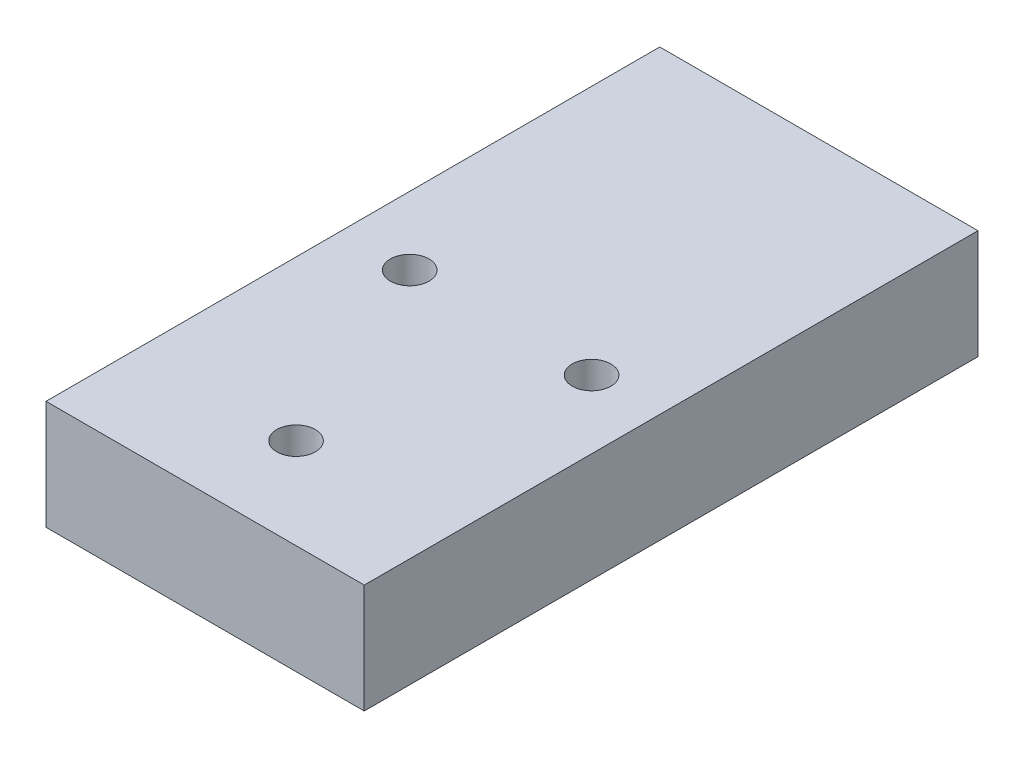
from build123d import *

# Parameters (mm, degrees)
SKETCH_1_W          = 70
SKETCH_1_H          = 135
EXTRUDE_1_DEPTH     = 24
HOLE_WIZARD_M10_1_D = 8.5


with BuildPart() as part:
    # 草图1 → 凸台-拉伸1 (new body)
    with BuildSketch(Plane(origin=(0, 0, 0), x_dir=(1, 0, 0), z_dir=(0, 1, 0))):
        Rectangle(SKETCH_1_W, SKETCH_1_H)
    extrude(amount=EXTRUDE_1_DEPTH)

    # M10 螺纹孔1 (through all)
    with Locations(Plane(origin=(0, 24, 0), x_dir=(1, 0, 0), z_dir=(0, 1, 0))):
        with Locations((-20, -2.5), (20, -2.5), (0, -47.5)):
            Hole(HOLE_WIZARD_M10_1_D / 2)


solid = part.part
